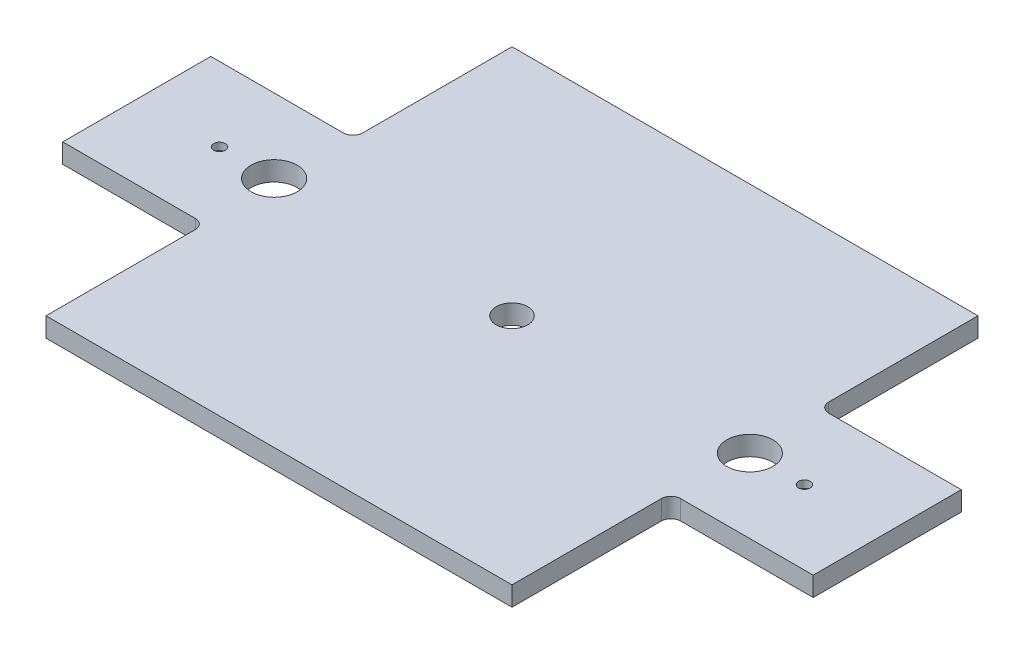
from build123d import *

# Parameters (mm, degrees)
EXTRUDE_1_DEPTH           = 40
SKETCH_2_R                = 20
CUT_EXTRUDE_1_DEPTH       = 10
HOLE_WIZARD_0_D           = 15.5
HOLE_WIZARD_0_CBORE_D     = 24
HOLE_WIZARD_0_CBORE_DEPTH = 15
SKETCH_5_R                = 47.5
CUT_EXTRUDE_2_DEPTH       = 911.7848264
SKETCH_6_R                = 32.5
CUT_EXTRUDE_3_DEPTH       = 911.7848264
FILLET_1_R                = 20


with BuildPart() as part:
    # 草图1 → 凸台-拉伸1 (new body)
    with BuildSketch(Plane(origin=(0, 0, 0), x_dir=(1, 0, 0), z_dir=(0, 1, 0))):
        Polygon((-480, 480), (480, 480), (480, 152.5), (773, 152.5), (773, -152.5), (480, -152.5), (480, -480), (-480, -480), (-480, -152.5), (-773, -152.5), (-773, 152.5), (-480, 152.5), align=None)
    extrude(amount=EXTRUDE_1_DEPTH)

    # 草图2 → 切除-拉伸1 (cut)
    with BuildSketch(Plane.XZ):
        with Locations(Location((602.5, 0, 0), (0, 0, 270))):
            Circle(SKETCH_2_R)
    cut_extrude_1 = extrude(amount=-CUT_EXTRUDE_1_DEPTH, mode=Mode.SUBTRACT)

    # 打孔尺寸(%根据)内六角圆柱头螺钉的类型0 (through all)
    with Locations(Plane(origin=(0, 40, 0), x_dir=(1, 0, 0), z_dir=(0, 1, 0))):
        with Locations((602.5, 0)):
            hole_wizard_0 = CounterBoreHole(HOLE_WIZARD_0_D / 2, HOLE_WIZARD_0_CBORE_D / 2, HOLE_WIZARD_0_CBORE_DEPTH)

    # 镜向1: 切除-拉伸1, 打孔尺寸(%根据)内六角圆柱头螺钉的类型0 across plane
    add(cut_extrude_1.mirror(Plane(origin=(0, 0, 0), x_dir=(0, 0, 1), z_dir=(1, 0, 0))), mode=Mode.SUBTRACT)
    add(hole_wizard_0.mirror(Plane(origin=(0, 0, 0), x_dir=(0, 0, 1), z_dir=(1, 0, 0))), mode=Mode.SUBTRACT)

    # 草图5 → 切除-拉伸2 (cut, through all)
    with BuildSketch(Plane.XZ):
        with Locations(Location((490, 0, 0), (0, 0, 270))):
            Circle(SKETCH_5_R)
    cut_extrude_2 = extrude(amount=-CUT_EXTRUDE_2_DEPTH, mode=Mode.SUBTRACT)

    # 镜向2: 切除-拉伸2 across plane
    add(cut_extrude_2.mirror(Plane(origin=(0, 0, 0), x_dir=(0, 0, 1), z_dir=(1, 0, 0))), mode=Mode.SUBTRACT)

    # 草图6 → 切除-拉伸3 (cut, through all)
    with BuildSketch(Plane(origin=(0, 40, 0), x_dir=(1, 0, 0), z_dir=(0, 1, 0))):
        with Locations(Location((0, 0, 0), (0, 0, 270))):
            Circle(SKETCH_6_R)
    extrude(amount=-CUT_EXTRUDE_3_DEPTH, mode=Mode.SUBTRACT)

    # 圆角1
    fillet_1_edges = [part.edges().sort_by_distance(p)[0] for p in [
        (-480, 20, 152.5),
        (-480, 20, -152.5),
        (480, 20, -152.5),
        (480, 20, 152.5),
    ]]
    fillet(fillet_1_edges, radius=FILLET_1_R)


solid = part.part
